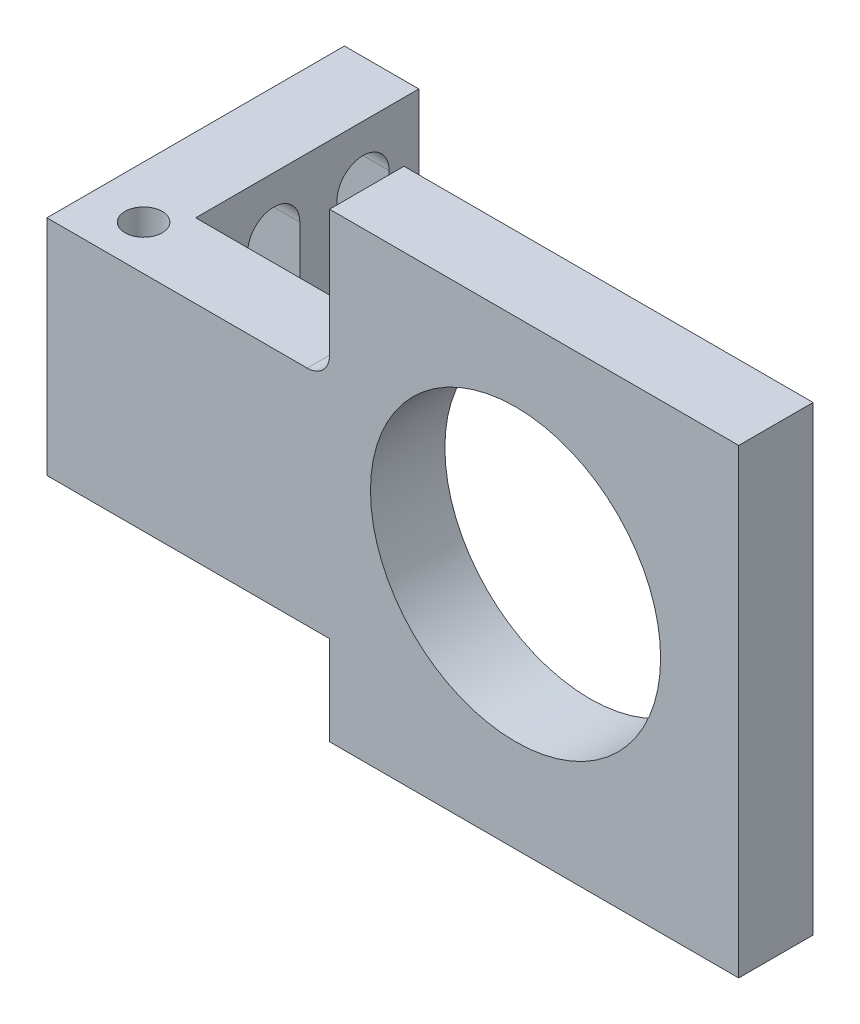
from build123d import *

# Parameters (mm, degrees)
EXTRUDE_1_DEPTH        = 5
FILLET_1_R             = 3
CUT_EXTRUDE_1_REACH    = 77
SKETCH_2_R             = 19.5
SKETCH_4_W             = 10
SKETCH_4_H             = 30
EXTRUDE_2_DEPTH        = 30
CUT_EXTRUDE_3_REACH    = 105.024
HOLE_WIZARD_M6_1_D     = 5
HOLE_WIZARD_M6_1_DEPTH = 15
HOLE_WIZARD_M6_1_TIP   = 1.502151548
SKETCH_7_W             = 55
SKETCH_7_H             = 10
EXTRUDE_3_DEPTH        = 12


with BuildPart() as part:
    # 草图1 → 凸台-拉伸1 (new, symmetric)
    with BuildSketch(Plane.XY):
        Polygon((0, 0), (55, 0), (55, -50), (-38, -50), (-38, -20), (0, -20), align=None)
    extrude(amount=EXTRUDE_1_DEPTH, both=True)

    # 圆角1
    fillet_1_edges = [part.edges().sort_by_distance(p)[0] for p in [
        (0, -20, 0),
    ]]
    fillet(fillet_1_edges, radius=FILLET_1_R)

    # 草图2 → 切除-拉伸1 (cut, up to next)
    with BuildSketch(Plane(origin=(0, 0, -5), x_dir=(-1, 0, 0), z_dir=(0, 0, -1)), mode=Mode.PRIVATE) as cut_extrude_1_sk1:
        with Locations((-25, -30)):
            Circle(SKETCH_2_R)
    cut_extrude_1_tool1 = extrude(cut_extrude_1_sk1.sketch, amount=-CUT_EXTRUDE_1_REACH, mode=Mode.PRIVATE) & part.part
    add(cut_extrude_1_tool1.solids().sort_by_distance((25, -30, -5))[0], mode=Mode.SUBTRACT)

    # 草图4 → 凸台-拉伸2 (add)
    with BuildSketch(Plane(origin=(0, 0, -5), x_dir=(-1, 0, 0), z_dir=(0, 0, -1))):
        with Locations((33, -35)):
            Rectangle(SKETCH_4_W, SKETCH_4_H)
    extrude(amount=EXTRUDE_2_DEPTH)

    # 草图5 → 切除-拉伸3 (cut, up to next)
    with BuildSketch(Plane(origin=(-28, 0, 0), x_dir=(0, 0, -1), z_dir=(1, 0, 0)), mode=Mode.PRIVATE) as cut_extrude_3_sk1:
        with BuildLine():
            Line((31, -27.5), (31, -42.5))
            ThreePointArc((31, -42.5), (27.5, -46), (24, -42.5))
            Line((24, -42.5), (24, -27.5))
            ThreePointArc((24, -27.5), (27.5, -24), (31, -27.5))
        make_face()
    cut_extrude_3_tool1 = extrude(cut_extrude_3_sk1.sketch, amount=-CUT_EXTRUDE_3_REACH, mode=Mode.PRIVATE) & part.part
    # 草图5 → 切除-拉伸3 (cut, up to next)
    with BuildSketch(Plane(origin=(-28, 0, 0), x_dir=(0, 0, -1), z_dir=(1, 0, 0)), mode=Mode.PRIVATE) as cut_extrude_3_sk2:
        with BuildLine():
            Line((19, -27.5), (19, -42.5))
            ThreePointArc((19, -42.5), (15.5, -46), (12, -42.5))
            Line((12, -42.5), (12, -27.5))
            ThreePointArc((12, -27.5), (15.5, -24), (19, -27.5))
        make_face()
    cut_extrude_3_tool2 = extrude(cut_extrude_3_sk2.sketch, amount=-CUT_EXTRUDE_3_REACH, mode=Mode.PRIVATE) & part.part
    add(cut_extrude_3_tool1.solids().sort_by_distance((-28, -35, -27.5))[0], mode=Mode.SUBTRACT)
    add(cut_extrude_3_tool2.solids().sort_by_distance((-28, -35, -15.5))[0], mode=Mode.SUBTRACT)

    # M6 螺纹孔1
    with Locations(Plane(origin=(-31, -20, -1), x_dir=(0, 0, 1), z_dir=(0, 1, 0))):
        with Locations((0, 0)):
            Hole(HOLE_WIZARD_M6_1_D / 2, depth=HOLE_WIZARD_M6_1_DEPTH)
            with Locations((0, 0, -(HOLE_WIZARD_M6_1_DEPTH + HOLE_WIZARD_M6_1_TIP / 2))):  # 118° drill point
                Cone(0, HOLE_WIZARD_M6_1_D / 2, HOLE_WIZARD_M6_1_TIP, mode=Mode.SUBTRACT)

    # 草图7 → 凸台-拉伸3 (add)
    with BuildSketch(Plane.XZ.offset(50)):
        with Locations((27.5, 0)):
            Rectangle(SKETCH_7_W, SKETCH_7_H)
    extrude(amount=EXTRUDE_3_DEPTH)


solid = part.part
